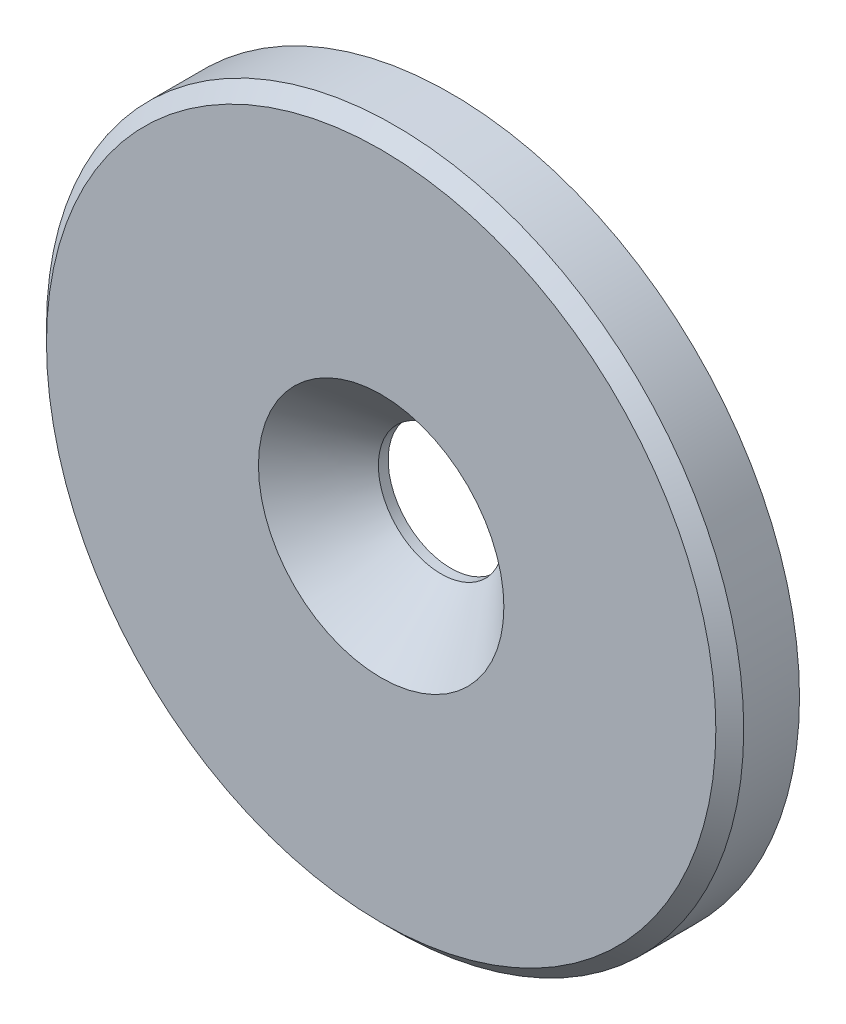
from build123d import *

# Parameters (mm, degrees)
SKETCH_1_R      = 25
EXTRUDE_1_DEPTH = 5
CHAMFER_1_SIZE  = 1


with BuildPart() as part:
    # 草图1 → 凸台-拉伸1 (new body)
    with BuildSketch(Plane.XY):
        Circle(SKETCH_1_R)
    extrude(amount=EXTRUDE_1_DEPTH)

    # 草图3 → 打孔尺寸(%根据)内六角花形半沉头螺钉的类型1 (revolve, cut)
    with BuildSketch(Plane(origin=(0, 0, 5), x_dir=(0, -1, 0), z_dir=(1, 0, 0))):
        Polygon((0, 0), (0, 5), (4.5, 5), (4.5, 4.3), (8.8, 0), align=None)
    revolve(axis=Axis((0, 0, 11.35), (0, 0, -1)), mode=Mode.SUBTRACT)

    # 倒角1
    chamfer_1_edges = [part.edges().sort_by_distance(p)[0] for p in [
        (-25, 0, 5),
    ]]
    chamfer(chamfer_1_edges, length=CHAMFER_1_SIZE)


solid = part.part
